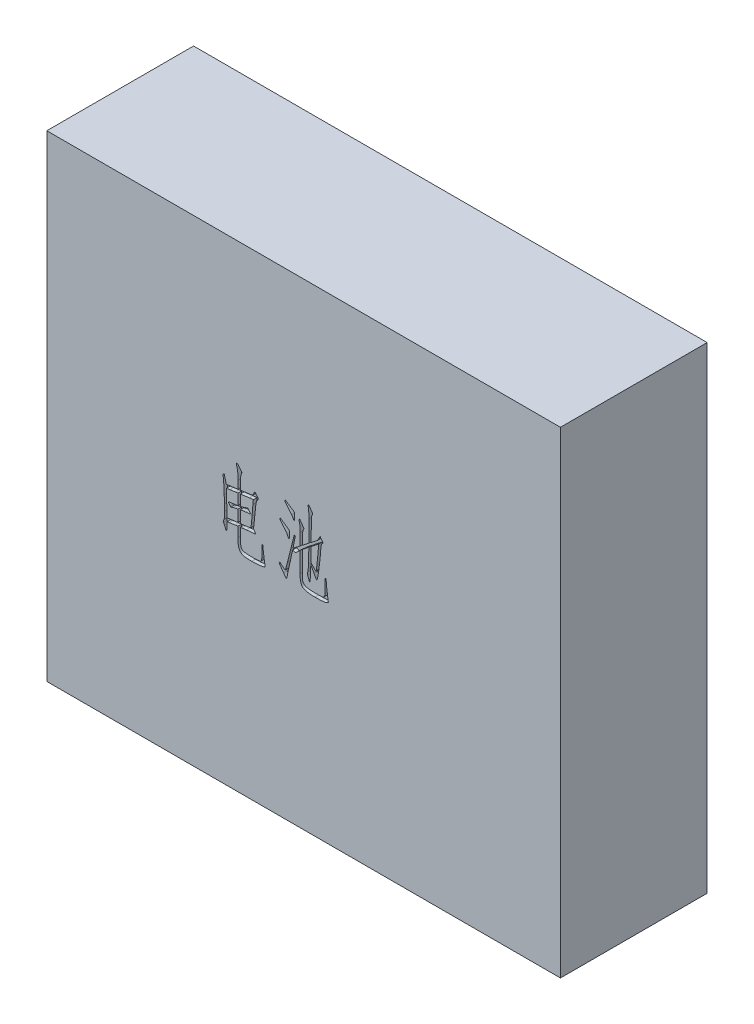
from build123d import *

# Parameters (mm, degrees)
SKETCH1_W           = 70
SKETCH1_H           = 65
BOSS_EXTRUDE1_DEPTH = 20
CUT_EXTRUDE1_DEPTH  = 0.5


with BuildPart() as part:
    # Sketch1 → Boss-Extrude1 (new body)
    with BuildSketch(Plane.XY):
        with Locations((-35, 32.5)):
            Rectangle(SKETCH1_W, SKETCH1_H)
    extrude(amount=BOSS_EXTRUDE1_DEPTH)

    # Sketch2 → Cut-Extrude1 (cut)
    # profile 1 of 4: a face of its own
    with BuildSketch(Plane.XY.offset(20)):
        with BuildLine():
            Line((-45.812964471, 36.577951622), (-45.662953817, 36.013707002))
            Line((-45.662953817, 36.013707002), (-45.536808494, 35.51935371))
            Line((-45.536808494, 35.51935371), (-45.100413864, 35.565379706))
            Line((-45.100413864, 35.565379706), (-44.179893941, 35.679592363))
            Line((-44.179893941, 35.679592363), (-43.937831294, 35.72561836))
            Line((-43.937831294, 35.72561836), (-43.925898629, 36.784216271))
            add(Edge.make_bspline(
                [(-43.925898629, 36.784216271), (-43.925848472, 36.793308603), (-43.925691689, 36.821730497), (-43.928371074, 36.879661448), (-43.929044334, 36.96833947), (-43.933127204, 37.085947103), (-43.937193687, 37.229243594), (-43.947978078, 37.394055669), (-43.963557741, 37.578165031), (-43.983093329, 37.777875129), (-44.010364708, 37.986611595), (-44.052989031, 38.195650038), (-44.109621861, 38.401561451), (-44.15640205, 38.535722825), (-44.179893941, 38.603095453)],
                knots=[0, 0, 0, 0, 0.177294891, 0.554209453, 1.130524385, 1.906506064, 2.848971625, 3.925876191, 5.126764862, 6.452083082, 7.83897123, 9.22979357, 10.608868701, 12, 12, 12, 12], degree=3))
            Line((-44.179893941, 38.603095453), (-44.075909283, 38.763334106))
            Line((-44.075909283, 38.763334106), (-43.38551934, 37.980892172))
            add(Edge.make_bspline(
                [(-43.38551934, 37.980892172), (-43.420264988, 37.902053364), (-43.488395113, 37.747464282), (-43.548848415, 37.540251846), (-43.578172835, 37.355960049), (-43.591770735, 37.182751904), (-43.60237328, 36.972995597), (-43.603245164, 36.820601132), (-43.603716655, 36.738190275)],
                knots=[0, 0, 0, 0, 1.215957117, 2.384278755, 3.034624226, 3.848266097, 4.836399765, 6, 6, 6, 6], degree=3))
            Line((-43.603716655, 36.738190275), (-43.603716655, 35.771644356))
            Line((-43.603716655, 35.771644356), (-43.039472036, 35.841535683))
            Line((-43.039472036, 35.841535683), (-42.154750109, 35.967681006))
            Line((-42.154750109, 35.967681006), (-41.934848128, 36.013707002))
            Line((-41.934848128, 36.013707002), (-41.740516144, 36.416008302))
            add(Edge.make_bspline(
                [(-41.740516144, 36.416008302), (-41.731928078, 36.435064247), (-41.717356021, 36.467397986), (-41.693448368, 36.504929362), (-41.679441503, 36.530548341), (-41.658607454, 36.540135813), (-41.639691378, 36.525794581), (-41.615948836, 36.50712574), (-41.581405092, 36.478434132), (-41.55779387, 36.453777511), (-41.544479494, 36.439873633)],
                knots=[0, 0, 0, 0, 1.663720426, 2.822966936, 3.56700533, 3.954602535, 4.461796658, 5.269494342, 6.4602669, 8, 8, 8, 8], degree=3))
            Line((-41.544479494, 36.439873633), (-41.268323517, 36.129624326))
            add(Edge.make_bspline(
                [(-41.268323517, 36.129624326), (-41.255200499, 36.111510287), (-41.231452655, 36.078730527), (-41.200612861, 36.034289255), (-41.185844914, 35.994837324), (-41.180962255, 35.955454126), (-41.18988266, 35.917798696), (-41.202635799, 35.882495715), (-41.225111729, 35.850918255), (-41.252022896, 35.807221487), (-41.292648636, 35.744473992), (-41.348482267, 35.664851326), (-41.405037234, 35.561917373), (-41.449581952, 35.433292488), (-41.487298387, 35.283335175), (-41.502389125, 35.174648675), (-41.510386163, 35.11705241)],
                knots=[0, 0, 0, 0, 0.847429402, 1.533536147, 2.036930199, 2.426382901, 3.016860564, 3.480069352, 3.837966044, 4.476237987, 5.424607541, 6.665143789, 8.156530738, 9.850434346, 11.801019622, 14, 14, 14, 14], degree=3))
            Line((-41.510386163, 35.11705241), (-41.636531486, 33.92037651))
            Line((-41.636531486, 33.92037651), (-41.78654214, 32.457772632))
            Line((-41.78654214, 32.457772632), (-41.832568136, 32.089564663))
            Line((-41.832568136, 32.089564663), (-41.612666155, 31.779315355))
            add(Edge.make_bspline(
                [(-41.612666155, 31.779315355), (-41.597709173, 31.753286049), (-41.572966997, 31.710227784), (-41.555564052, 31.64939674), (-41.572704739, 31.601362265), (-41.59930459, 31.597267994), (-41.612666155, 31.59521137)],
                knots=[0, 0, 0, 0, 1.606901506, 2.658172752, 3.325977029, 4, 4, 4, 4], degree=3))
            Line((-41.612666155, 31.59521137), (-41.796770139, 31.583278705))
            Line((-41.796770139, 31.583278705), (-42.809342055, 31.491226712))
            Line((-42.809342055, 31.491226712), (-43.38551934, 31.423040051))
            Line((-43.38551934, 31.423040051), (-43.627581987, 31.388946721))
            Line((-43.627581987, 31.388946721), (-43.627581987, 30.146244824))
            add(Edge.make_bspline(
                [(-43.627581987, 30.146244824), (-43.625455316, 30.020075821), (-43.621338914, 29.775861911), (-43.598644778, 29.477145058), (-43.561803409, 29.256634492), (-43.518466195, 29.109417545), (-43.454741682, 28.980941201), (-43.39204268, 28.878371677), (-43.308783505, 28.812143731), (-43.214226104, 28.772149677), (-43.089428354, 28.736815118), (-42.932276864, 28.709423108), (-42.742740398, 28.687794227), (-42.521412057, 28.673764216), (-42.267931823, 28.6629308), (-42.088282823, 28.661983652), (-41.99280679, 28.661480282)],
                knots=[0, 0, 0, 0, 1.931152807, 3.737957541, 4.577172512, 5.350113142, 6.073531508, 6.773090527, 7.162848559, 7.680298175, 8.332476513, 9.14602524, 10.117846342, 11.250994603, 12.539017008, 14, 14, 14, 14], degree=3))
            add(Edge.make_bspline(
                [(-41.99280679, 28.661480282), (-41.903594337, 28.661133851), (-41.735947315, 28.660482842), (-41.501154339, 28.664711566), (-41.29978544, 28.676356186), (-41.132131419, 28.693113532), (-40.996618699, 28.712927385), (-40.895964252, 28.741581905), (-40.822055206, 28.771883437), (-40.756217937, 28.857328089), (-40.726796655, 29.002470979), (-40.711695577, 29.127077752), (-40.704078897, 29.189926904)],
                knots=[0, 0, 0, 0, 1.652015129, 3.104447941, 4.3482727, 5.384821521, 6.227270062, 6.873348196, 7.334536251, 7.663266203, 8.821398446, 10, 10, 10, 10], degree=3))
            Line((-40.704078897, 29.189926904), (-40.704078897, 29.824062851))
            Line((-40.704078897, 29.824062851), (-40.704078897, 30.824702101))
            Line((-40.704078897, 30.824702101), (-40.566000909, 30.846862766))
            Line((-40.566000909, 30.846862766), (-40.543840244, 30.570706789))
            Line((-40.543840244, 30.570706789), (-40.485881582, 30.100218828))
            Line((-40.485881582, 30.100218828), (-40.405762255, 29.478015547))
            Line((-40.405762255, 29.478015547), (-40.323938262, 28.949568924))
            Line((-40.323938262, 28.949568924), (-40.267684267, 28.569428289))
            add(Edge.make_bspline(
                [(-40.267684267, 28.569428289), (-40.261677644, 28.537454545), (-40.252021936, 28.486056413), (-40.248582565, 28.417397749), (-40.27837879, 28.372014815), (-40.307431463, 28.358761234), (-40.323938262, 28.351230974)],
                knots=[0, 0, 0, 0, 1.559608042, 2.507086382, 3.151774227, 4, 4, 4, 4], degree=3))
            Line((-40.323938262, 28.351230974), (-40.415990254, 28.315432977))
            add(Edge.make_bspline(
                [(-40.415990254, 28.315432977), (-40.426712478, 28.311220837), (-40.452204778, 28.30120639), (-40.49889938, 28.290668166), (-40.558255604, 28.276259718), (-40.631918341, 28.263690168), (-40.718618541, 28.24755137), (-40.818903004, 28.233306325), (-40.932319784, 28.215269905), (-41.185704737, 28.182282751), (-41.567309043, 28.143795243), (-41.907463787, 28.143436273), (-42.072926116, 28.143261658)],
                knots=[0, 0, 0, 0, 0.206618915, 0.491240576, 0.857597671, 1.30390666, 1.832361082, 2.441372039, 3.122534554, 3.89462094, 7.030145068, 10, 10, 10, 10], degree=3))
            add(Edge.make_bspline(
                [(-42.072926116, 28.143261658), (-42.164420521, 28.143842078), (-42.337813117, 28.144942042), (-42.583433704, 28.154993204), (-42.800723206, 28.171504943), (-42.990269829, 28.194753914), (-43.152856969, 28.224574619), (-43.287782923, 28.261157691), (-43.396097067, 28.303323646), (-43.497889486, 28.372667533), (-43.591364505, 28.467455716), (-43.686841354, 28.578088586), (-43.76197096, 28.688945914), (-43.832245139, 28.844347638), (-43.885969719, 29.060569894), (-43.931062669, 29.343564055), (-43.955099128, 29.656034013), (-43.958331496, 29.872898525), (-43.959991959, 29.984301505)],
                knots=[0, 0, 0, 0, 1.375107078, 2.605988713, 3.693973982, 4.649466436, 5.475237603, 6.17560074, 6.749778481, 7.211670088, 8.015056038, 8.742243092, 9.407844955, 10.019243034, 11.295622579, 12.740386124, 14.325541172, 16, 16, 16, 16], degree=3))
            Line((-43.959991959, 29.984301505), (-43.959991959, 31.342920725))
            Line((-43.959991959, 31.342920725), (-44.306039264, 31.307122728))
            Line((-44.306039264, 31.307122728), (-45.134507194, 31.180977405))
            Line((-45.134507194, 31.180977405), (-45.432823836, 31.134951409))
            Line((-45.432823836, 31.134951409), (-45.444756502, 30.616732785))
            Line((-45.444756502, 30.616732785), (-45.456689168, 30.318416143))
            add(Edge.make_bspline(
                [(-45.456689168, 30.318416143), (-45.458359636, 30.273533328), (-45.461551521, 30.187772505), (-45.487511175, 30.102103524), (-45.51112075, 30.029386641), (-45.558375641, 30.038317065), (-45.586013212, 30.089408838), (-45.604968918, 30.130530018), (-45.616927821, 30.156472824)],
                knots=[0, 0, 0, 0, 1.721263003, 3.288940973, 3.839377096, 4.198736227, 4.863606649, 6, 6, 6, 6], degree=3))
            Line((-45.616927821, 30.156472824), (-45.790803806, 30.548546124))
            Line((-45.790803806, 30.548546124), (-45.905016464, 30.80083677))
            add(Edge.make_bspline(
                [(-45.905016464, 30.80083677), (-45.916225525, 30.826818695), (-45.934025264, 30.86807741), (-45.962588158, 30.920163424), (-45.950434446, 30.967100334), (-45.933584803, 31.023789903), (-45.899924863, 31.10577543), (-45.873762283, 31.169092752), (-45.858990467, 31.204842736)],
                knots=[0, 0, 0, 0, 1.195724136, 1.898783123, 2.330290027, 3.145663464, 4.388395428, 6, 6, 6, 6], degree=3))
            add(Edge.make_bspline(
                [(-45.858990467, 31.204842736), (-45.849809434, 31.226217303), (-45.830217739, 31.271829156), (-45.812969093, 31.350842435), (-45.798550733, 31.441839518), (-45.794928356, 31.578213425), (-45.791037076, 31.745202497), (-45.786619115, 31.927653626), (-45.780327837, 32.074186752), (-45.779294197, 32.158883823), (-45.778871141, 32.193549321)],
                knots=[0, 0, 0, 0, 0.558699634, 1.192226558, 1.938775613, 2.774002823, 4.470288396, 5.961506424, 7.165668957, 8, 8, 8, 8], degree=3))
            Line((-45.778871141, 32.193549321), (-45.790803806, 33.056110582))
            Line((-45.790803806, 33.056110582), (-45.824897137, 34.138573825))
            add(Edge.make_bspline(
                [(-45.824897137, 34.138573825), (-45.824797251, 34.152212755), (-45.824559958, 34.184613823), (-45.827034133, 34.2397075), (-45.828061889, 34.308497074), (-45.831764637, 34.390323987), (-45.837314584, 34.486300534), (-45.842238946, 34.595980451), (-45.846952964, 34.719327295), (-45.856167901, 34.894310057), (-45.866887814, 35.102277761), (-45.877722314, 35.324559799), (-45.890900336, 35.502261385), (-45.899135518, 35.652460744), (-45.913678834, 35.80572857), (-45.929393585, 35.994614848), (-45.956882817, 36.234104167), (-45.975113007, 36.410873963), (-45.98513579, 36.508060294)],
                knots=[0, 0, 0, 0, 0.275532466, 0.654563513, 1.113927774, 1.665470852, 2.30930182, 3.056329963, 3.883644582, 4.803233469, 6.596547928, 8.091177521, 9.299307877, 10.196626331, 11.130014446, 12.409513054, 14.025984863, 16, 16, 16, 16], degree=3))
            Line((-45.98513579, 36.508060294), (-45.812964471, 36.577951622))
        make_face()
        with BuildLine():
            Line((-45.432823836, 31.607144036), (-43.959991959, 31.779315355))
            Line((-43.959991959, 31.779315355), (-43.94976396, 33.378292555))
            Line((-43.94976396, 33.378292555), (-44.260013267, 33.310105894))
            Line((-44.260013267, 33.310105894), (-44.616288571, 33.218053902))
            Line((-44.616288571, 33.218053902), (-44.938470544, 33.102136578))
            Line((-44.938470544, 33.102136578), (-45.018589871, 33.218053902))
            Line((-45.018589871, 33.218053902), (-45.214626521, 33.470344547))
            add(Edge.make_bspline(
                [(-45.214626521, 33.470344547), (-45.22660598, 33.483568984), (-45.247192553, 33.506295039), (-45.261151514, 33.549702385), (-45.239906849, 33.586199824), (-45.215591355, 33.594037338), (-45.202693855, 33.598194537)],
                knots=[0, 0, 0, 0, 1.284117706, 2.206742812, 3.048814964, 4, 4, 4, 4], degree=3))
            Line((-45.202693855, 33.598194537), (-44.800392556, 33.654448532))
            Line((-44.800392556, 33.654448532), (-44.328199928, 33.712407194))
            Line((-44.328199928, 33.712407194), (-43.94976396, 33.782298521))
            Line((-43.94976396, 33.782298521), (-43.937831294, 35.277291064))
            Line((-43.937831294, 35.277291064), (-44.282173932, 35.219332402))
            Line((-44.282173932, 35.219332402), (-45.054387868, 35.11705241))
            Line((-45.054387868, 35.11705241), (-45.524875829, 35.035228417))
            Line((-45.524875829, 35.035228417), (-45.502715164, 34.138573825))
            Line((-45.502715164, 34.138573825), (-45.432823836, 31.607144036))
        make_face(mode=Mode.SUBTRACT)
        with BuildLine():
            Line((-43.627581987, 31.825341351), (-42.799114056, 31.917393344))
            Line((-42.799114056, 31.917393344), (-42.407040755, 31.987284671))
            Line((-42.407040755, 31.987284671), (-42.176910774, 32.033310667))
            Line((-42.176910774, 32.033310667), (-42.118952112, 32.585622621))
            Line((-42.118952112, 32.585622621), (-42.02690012, 33.516370544))
            Line((-42.02690012, 33.516370544), (-41.912687463, 34.92101576))
            Line((-41.912687463, 34.92101576), (-41.854728801, 35.531286376))
            Line((-41.854728801, 35.531286376), (-42.395108089, 35.473327714))
            Line((-42.395108089, 35.473327714), (-43.615649321, 35.311384394))
            Line((-43.615649321, 35.311384394), (-43.627581987, 33.850485182))
            add(Edge.make_bspline(
                [(-43.627581987, 33.850485182), (-43.518158759, 33.876588548), (-43.314629368, 33.925141329), (-43.03688824, 34.009381589), (-42.805865185, 34.08904511), (-42.674156189, 34.154987357), (-42.615010071, 34.184599821)],
                knots=[0, 0, 0, 0, 1.262396956, 2.348083582, 3.25817942, 4, 4, 4, 4], degree=3))
            Line((-42.615010071, 34.184599821), (-42.303056097, 33.804459186))
            add(Edge.make_bspline(
                [(-42.303056097, 33.804459186), (-42.287987807, 33.780864519), (-42.262053617, 33.740255495), (-42.244999942, 33.678242919), (-42.26725058, 33.626405214), (-42.298551095, 33.6224384), (-42.314988763, 33.620355202)],
                knots=[0, 0, 0, 0, 1.442479735, 2.482666664, 3.203162602, 4, 4, 4, 4], degree=3))
            Line((-42.314988763, 33.620355202), (-42.476932083, 33.608422536))
            Line((-42.476932083, 33.608422536), (-42.855368051, 33.56239654))
            Line((-42.855368051, 33.56239654), (-43.22357602, 33.516370544))
            Line((-43.22357602, 33.516370544), (-43.627581987, 33.436251217))
            Line((-43.627581987, 33.436251217), (-43.627581987, 31.825341351))
        make_face(mode=Mode.SUBTRACT)
    # profile 2 of 4: a face of its own
    with BuildSketch(Plane.XY.offset(20)):
        with BuildLine():
            Line((-36.266831933, 34.16073449), (-36.128753945, 34.092547829))
            Line((-36.128753945, 34.092547829), (-36.198645272, 33.75843319))
            Line((-36.198645272, 33.75843319), (-36.450935918, 32.503798628))
            Line((-36.450935918, 32.503798628), (-35.474162, 33.240214567))
            Line((-35.474162, 33.240214567), (-35.474162, 34.874989764))
            add(Edge.make_bspline(
                [(-35.474162, 34.874989764), (-35.476014604, 34.96137645), (-35.479489325, 35.123402178), (-35.490539761, 35.349501037), (-35.500546316, 35.543024737), (-35.524060765, 35.755403005), (-35.560200686, 35.996883008), (-35.617784828, 36.177939791), (-35.646333318, 36.267702314)],
                knots=[0, 0, 0, 0, 1.103429514, 2.069577835, 2.891178562, 3.577175633, 4.798836336, 6, 6, 6, 6], degree=3))
            Line((-35.646333318, 36.267702314), (-35.54234866, 36.405780303))
            Line((-35.54234866, 36.405780303), (-34.955943376, 35.577312372))
            add(Edge.make_bspline(
                [(-34.955943376, 35.577312372), (-34.974187002, 35.535505071), (-35.008613632, 35.456612614), (-35.047899028, 35.341111526), (-35.084247663, 35.239951635), (-35.111919704, 35.121866565), (-35.134793499, 34.98830644), (-35.148705642, 34.833197358), (-35.151718217, 34.673813064), (-35.156499279, 34.53809038), (-35.158834538, 34.433999815), (-35.159376391, 34.376731057), (-35.157831897, 34.341522739), (-35.153209175, 34.326636069), (-35.151980026, 34.32267781)],
                knots=[0, 0, 0, 0, 1.277874718, 2.411413148, 3.418754168, 4.287932458, 5.8066473, 7.214043668, 8.648311221, 10.273614673, 11.022374716, 11.563908357, 11.884046341, 12, 12, 12, 12], degree=3))
            Line((-35.151980026, 34.32267781), (-35.151980026, 33.506142545))
            Line((-35.151980026, 33.506142545), (-34.287714098, 34.172667156))
            Line((-34.287714098, 34.172667156), (-34.265553434, 37.060372248))
            add(Edge.make_bspline(
                [(-34.265553434, 37.060372248), (-34.265567288, 37.080828343), (-34.265606541, 37.138787278), (-34.265162028, 37.226295863), (-34.266854845, 37.335473149), (-34.275011468, 37.46155569), (-34.28448686, 37.625286771), (-34.299716924, 37.815015709), (-34.315236821, 38.006585831), (-34.331193271, 38.175590104), (-34.350006539, 38.309063556), (-34.363687497, 38.386063025), (-34.369538092, 38.418991468)],
                knots=[0, 0, 0, 0, 0.449890352, 1.274689332, 1.924651104, 2.850775754, 4.052824256, 5.531747845, 7.036580408, 8.280074453, 9.264482312, 10, 10, 10, 10], degree=3))
            Line((-34.369538092, 38.418991468), (-34.415564088, 38.625256118))
            Line((-34.415564088, 38.625256118), (-34.287714098, 38.68321478))
            Line((-34.287714098, 38.68321478), (-33.74733481, 37.900772845))
            add(Edge.make_bspline(
                [(-33.74733481, 37.900772845), (-33.766404625, 37.866289513), (-33.802202035, 37.801558211), (-33.847870249, 37.707751639), (-33.878165259, 37.622902765), (-33.899502497, 37.543742215), (-33.908881892, 37.458884191), (-33.915467155, 37.359370748), (-33.918190644, 37.239371454), (-33.919045193, 37.152991043), (-33.919506129, 37.106398244)],
                knots=[0, 0, 0, 0, 1.143336114, 2.146243721, 3.022303475, 3.754005903, 4.518761241, 5.493636838, 6.648090788, 8, 8, 8, 8], degree=3))
            Line((-33.919506129, 37.106398244), (-33.955304126, 36.335888975))
            Line((-33.955304126, 36.335888975), (-33.977464791, 34.414729802))
            Line((-33.977464791, 34.414729802), (-33.068877533, 35.127280409))
            Line((-33.068877533, 35.127280409), (-32.872840883, 35.51935371))
            add(Edge.make_bspline(
                [(-32.872840883, 35.51935371), (-32.856433799, 35.552914195), (-32.82830764, 35.6104459), (-32.792135435, 35.682424601), (-32.770561775, 35.725618797), (-32.760901283, 35.744937997), (-32.758628226, 35.749483691)],
                knots=[0, 0, 0, 0, 1.744829883, 2.991108106, 3.762613672, 4, 4, 4, 4], degree=3))
            Line((-32.758628226, 35.749483691), (-32.676804233, 35.633566367))
            Line((-32.676804233, 35.633566367), (-32.458606917, 35.32331706))
            add(Edge.make_bspline(
                [(-32.458606917, 35.32331706), (-32.443653988, 35.302994829), (-32.417026915, 35.266806498), (-32.385056675, 35.218752815), (-32.365333603, 35.184146801), (-32.359121369, 35.156885985), (-32.368895301, 35.133542169), (-32.390568064, 35.110843652), (-32.415360258, 35.075245581), (-32.471571134, 35.026430074), (-32.533300526, 34.940260201), (-32.58332619, 34.817342596), (-32.613550103, 34.687073492), (-32.637155762, 34.574525941), (-32.647320913, 34.467048566), (-32.65797822, 34.35179159), (-32.667177907, 34.199368585), (-32.677326232, 34.048262427), (-32.685007695, 33.904931773), (-32.696276797, 33.776627085), (-32.707394313, 33.631611698), (-32.723623656, 33.469796301), (-32.740012444, 33.290688105), (-32.760661301, 33.094660481), (-32.784934581, 32.882253834), (-32.81776993, 32.583157902), (-32.86262768, 32.216139844), (-32.914711884, 31.797743919), (-32.967462662, 31.416422779), (-33.01173421, 31.123828042), (-33.047253659, 30.914378011), (-33.070368655, 30.781720304), (-33.093760988, 30.669020712), (-33.117931343, 30.576517991), (-33.139457992, 30.503551831), (-33.158917083, 30.449578549), (-33.178033124, 30.415054976), (-33.204460577, 30.392853951), (-33.241329818, 30.400660804), (-33.277931363, 30.424922015), (-33.313838902, 30.468260951), (-33.33381771, 30.504395439), (-33.34503351, 30.524680793)],
                knots=[0, 0, 0, 0, 0.572960633, 1.020286037, 1.308793021, 1.47849792, 1.629516928, 1.859238066, 2.189701376, 2.609377403, 3.540946753, 4.564231855, 5.603177511, 6.574893703, 7.171901031, 8.052674627, 9.203596934, 10.638611067, 11.491733585, 12.46250707, 13.562925808, 14.794144362, 16.155029084, 17.646864078, 19.269751124, 21.009474552, 24.479075422, 27.665373512, 30.5830622, 33.219864516, 34.384375344, 35.406846701, 36.277354076, 36.997119736, 37.576724451, 38.005620917, 38.295566847, 38.471058794, 38.743235739, 39.061902118, 39.473366081, 40, 40, 40, 40], degree=3))
            Line((-33.34503351, 30.524680793), (-33.587096157, 30.984940755))
            Line((-33.587096157, 30.984940755), (-33.885412799, 31.515092044))
            Line((-33.885412799, 31.515092044), (-34.023490787, 31.745222025))
            Line((-34.023490787, 31.745222025), (-34.057584118, 30.674691447))
            Line((-34.057584118, 30.674691447), (-34.103610114, 29.972368839))
            add(Edge.make_bspline(
                [(-34.103610114, 29.972368839), (-34.106429464, 29.934450286), (-34.111445377, 29.866989299), (-34.118331654, 29.776130099), (-34.136427813, 29.715454841), (-34.146112218, 29.667009521), (-34.189496201, 29.656430258), (-34.216489732, 29.713246126), (-34.251617239, 29.784219805), (-34.274228258, 29.851889453), (-34.287714098, 29.892249512)],
                knots=[0, 0, 0, 0, 1.548277697, 2.75454446, 3.632054474, 4.21957732, 4.527029857, 5.164410394, 6.308775526, 8, 8, 8, 8], degree=3))
            Line((-34.287714098, 29.892249512), (-34.449657418, 30.306483478))
            add(Edge.make_bspline(
                [(-34.449657418, 30.306483478), (-34.458630314, 30.329060699), (-34.474645019, 30.369356226), (-34.490058561, 30.424263975), (-34.504244789, 30.463715075), (-34.508970445, 30.495701665), (-34.504239928, 30.527686838), (-34.490277835, 30.566634975), (-34.47499331, 30.619937311), (-34.446190036, 30.684986815), (-34.419284066, 30.768308992), (-34.397550669, 30.872269511), (-34.381675766, 30.996582431), (-34.368686227, 31.135932694), (-34.3598749, 31.279274473), (-34.349848348, 31.414962542), (-34.347330571, 31.538381859), (-34.346206164, 31.616236764), (-34.34567276, 31.653170032)],
                knots=[0, 0, 0, 0, 0.847620795, 1.512822455, 1.989839709, 2.309771091, 2.629702473, 3.106719727, 3.753010358, 4.563594937, 5.586336595, 6.804437419, 8.266379239, 9.96034311, 11.690636616, 13.281037962, 14.71016275, 16, 16, 16, 16], degree=3))
            Line((-34.34567276, 31.653170032), (-34.287714098, 33.700474528))
            Line((-34.287714098, 33.700474528), (-35.151980026, 33.010084586))
            Line((-35.151980026, 33.010084586), (-35.174140691, 30.122379493))
            add(Edge.make_bspline(
                [(-35.174140691, 30.122379493), (-35.174140472, 30.115560828), (-35.17413987, 30.0968095), (-35.174148598, 30.059306784), (-35.174087003, 30.004757827), (-35.174429939, 29.931449836), (-35.172579481, 29.838797384), (-35.167835228, 29.723921765), (-35.155337701, 29.586034783), (-35.148882248, 29.430800344), (-35.119381123, 29.269799603), (-35.044165651, 29.122854344), (-34.931090073, 28.997709282), (-34.808317108, 28.912174159), (-34.688969348, 28.858162305), (-34.581804486, 28.820401233), (-34.459276254, 28.788287813), (-34.32118352, 28.763912688), (-34.168307845, 28.742717205), (-33.999787323, 28.730307966), (-33.815614193, 28.721514998), (-33.687683782, 28.720148965), (-33.621189487, 28.719438943)],
                knots=[0, 0, 0, 0, 0.160723151, 0.441988665, 0.883977329, 1.446508357, 2.169886539, 3.068156583, 4.156010134, 5.431851206, 6.732134165, 7.978026584, 9.268268598, 10.672745357, 11.469748722, 12.350880404, 13.348231265, 14.451557942, 15.654374443, 16.984662635, 18.432720347, 20, 20, 20, 20], degree=3))
            add(Edge.make_bspline(
                [(-33.621189487, 28.719438943), (-33.550731062, 28.718760795), (-33.416066642, 28.717464678), (-33.224562404, 28.717334614), (-33.052963938, 28.719256917), (-32.901155872, 28.721523233), (-32.769422857, 28.729529557), (-32.65725881, 28.734901764), (-32.565727993, 28.745197424), (-32.472846567, 28.759877815), (-32.380592014, 28.785778443), (-32.288133409, 28.821066771), (-32.219111079, 28.868162134), (-32.167579013, 28.924731454), (-32.138225494, 28.999698933), (-32.111878457, 29.08944655), (-32.099049201, 29.20219639), (-32.093446093, 29.283687485), (-32.090398948, 29.328004893)],
                knots=[0, 0, 0, 0, 1.766276756, 3.375815332, 4.800256971, 6.068266689, 7.180735551, 8.10832774, 8.882221105, 9.488708597, 10.463127887, 11.28049811, 11.956136324, 12.541689444, 13.166467087, 13.951035347, 14.885708911, 16, 16, 16, 16], degree=3))
            Line((-32.090398948, 29.328004893), (-32.090398948, 30.904821428))
            Line((-32.090398948, 30.904821428), (-32.090398948, 31.146884074))
            Line((-32.090398948, 31.146884074), (-31.95232096, 31.169044739))
            Line((-31.95232096, 31.169044739), (-31.906294963, 30.754810774))
            Line((-31.906294963, 30.754810774), (-31.848336302, 30.122379493))
            Line((-31.848336302, 30.122379493), (-31.722190979, 29.121740243))
            add(Edge.make_bspline(
                [(-31.722190979, 29.121740243), (-31.716410034, 29.071180568), (-31.706081299, 28.980846285), (-31.693670807, 28.861215467), (-31.680473943, 28.77363014), (-31.664727261, 28.700393767), (-31.647391817, 28.632678288), (-31.632702925, 28.570288193), (-31.643437061, 28.51575527), (-31.682937455, 28.478454086), (-31.738537519, 28.435842095), (-31.786920213, 28.411182678), (-31.814242971, 28.39725697)],
                knots=[0, 0, 0, 0, 1.862405269, 3.327534118, 4.401050164, 5.102555638, 6.065884989, 6.968735006, 7.417638403, 8.022127244, 8.88305229, 10, 10, 10, 10], degree=3))
            add(Edge.make_bspline(
                [(-31.814242971, 28.39725697), (-31.847473307, 28.382794897), (-31.9223428, 28.350211171), (-32.054525999, 28.316858225), (-32.215257185, 28.288611423), (-32.405445074, 28.265795085), (-32.624744914, 28.244856909), (-32.873836847, 28.231893647), (-33.151809015, 28.226061559), (-33.34673584, 28.224303485), (-33.449018168, 28.223380985)],
                knots=[0, 0, 0, 0, 0.525453063, 1.183870223, 1.971909494, 2.89486667, 3.96365597, 5.169900272, 6.514985356, 8, 8, 8, 8], degree=3))
            add(Edge.make_bspline(
                [(-33.449018168, 28.223380985), (-33.581475292, 28.223124504), (-33.833128402, 28.222637221), (-34.189161325, 28.252070607), (-34.503177112, 28.29961452), (-34.736660285, 28.358982933), (-34.899755786, 28.421003055), (-35.004939115, 28.476836508), (-35.099995186, 28.53868782), (-35.179742553, 28.61340677), (-35.249742785, 28.693428265), (-35.30437983, 28.784573832), (-35.349384388, 28.882593329), (-35.386342098, 29.019989162), (-35.41721705, 29.180048089), (-35.450264942, 29.347594644), (-35.472989564, 29.479358065), (-35.48959416, 29.602024959), (-35.492070822, 29.718379301), (-35.497044353, 29.829143167), (-35.496248969, 29.907024944), (-35.496303671, 29.947935712), (-35.496322664, 29.96214084)],
                knots=[0, 0, 0, 0, 2.462684528, 4.67881384, 6.636999054, 8.364825419, 9.147899839, 9.875905864, 10.576468373, 11.249712985, 11.901975396, 12.547265221, 13.219015024, 13.901323428, 15.186439089, 16.251823802, 17.077121389, 17.673568011, 18.551778676, 19.239061844, 19.735785362, 20, 20, 20, 20], degree=3))
            Line((-35.496322664, 29.96214084), (-35.474162, 32.72370061))
            add(Edge.make_bspline(
                [(-35.474162, 32.72370061), (-35.582177534, 32.63179892), (-35.795245885, 32.450516277), (-35.987793051, 32.247580367), (-36.082727949, 32.147523324)],
                knots=[0, 0, 0, 0, 1.013905004, 2, 2, 2, 2], degree=3))
            Line((-36.082727949, 32.147523324), (-36.496961914, 32.273668647))
            Line((-36.496961914, 32.273668647), (-36.808915888, 30.824702101))
            Line((-36.808915888, 30.824702101), (-37.165191192, 29.20185957))
            Line((-37.165191192, 29.20185957), (-37.233377853, 28.845584266))
            add(Edge.make_bspline(
                [(-37.233377853, 28.845584266), (-37.246794197, 28.787677115), (-37.269791443, 28.688417212), (-37.307409568, 28.556899267), (-37.324017813, 28.492978289), (-37.349845784, 28.441009346), (-37.372346316, 28.462343518), (-37.391314575, 28.486379095), (-37.42544239, 28.525943153), (-37.465087201, 28.581707099), (-37.519292286, 28.650562432), (-37.57882964, 28.738031645), (-37.651423725, 28.83848414), (-37.70225484, 28.910864763), (-37.729435812, 28.949568924)],
                knots=[0, 0, 0, 0, 2.07497586, 3.55676105, 4.466827747, 4.800211812, 4.968619417, 5.357211501, 5.941249148, 6.724328603, 7.73059332, 8.952705414, 10.370517209, 12, 12, 12, 12], degree=3))
            Line((-37.729435812, 28.949568924), (-38.257882434, 29.696212862))
            Line((-38.257882434, 29.696212862), (-38.349934427, 29.846223516))
            Line((-38.349934427, 29.846223516), (-38.281747766, 29.99623417))
            Line((-38.281747766, 29.99623417), (-38.165830442, 29.904182178))
            Line((-38.165830442, 29.904182178), (-37.775461808, 29.570067539))
            add(Edge.make_bspline(
                [(-37.775461808, 29.570067539), (-37.744311019, 29.54386298), (-37.689619759, 29.497855787), (-37.617952476, 29.432605449), (-37.569370165, 29.40477681), (-37.529600568, 29.369246809), (-37.507385765, 29.40848859), (-37.488548319, 29.456253362), (-37.458827166, 29.545320775), (-37.422995419, 29.665718967), (-37.375571655, 29.822434979), (-37.323927196, 30.0141315), (-37.264482481, 30.241110604), (-37.222004367, 30.403651067), (-37.199284522, 30.490587462)],
                knots=[0, 0, 0, 0, 1.003500883, 1.761840696, 2.269784058, 2.548928131, 2.726560793, 3.180073805, 3.912603369, 4.956880628, 6.27350926, 7.898819114, 9.806442298, 12, 12, 12, 12], degree=3))
            Line((-37.199284522, 30.490587462), (-36.370816591, 33.75843319))
            Line((-36.370816591, 33.75843319), (-36.266831933, 34.16073449))
        make_face()
        with BuildLine():
            Line((-34.023490787, 32.043538666), (-33.885412799, 31.895232679))
            add(Edge.make_bspline(
                [(-33.885412799, 31.895232679), (-33.842815042, 31.851459554), (-33.763223454, 31.769671854), (-33.651965646, 31.655920249), (-33.559776698, 31.557739713), (-33.479393502, 31.481373088), (-33.418611321, 31.41969568), (-33.371148497, 31.378891692), (-33.342193485, 31.352705851), (-33.325789623, 31.345071534), (-33.321168179, 31.342920725)],
                knots=[0, 0, 0, 0, 1.853692376, 3.463523279, 4.829501388, 5.939248689, 6.829515306, 7.452499084, 7.845753089, 8, 8, 8, 8], degree=3))
            add(Edge.make_bspline(
                [(-33.321168179, 31.342920725), (-33.318686316, 31.345660209), (-33.309435275, 31.35587152), (-33.30826821, 31.387061019), (-33.2944001, 31.431888441), (-33.289768994, 31.469402762), (-33.287074848, 31.491226712)],
                knots=[0, 0, 0, 0, 0.284593498, 1.060810166, 2.290126812, 4, 4, 4, 4], degree=3))
            Line((-33.287074848, 31.491226712), (-33.195022856, 32.067403998))
            add(Edge.make_bspline(
                [(-33.195022856, 32.067403998), (-33.192184436, 32.088428238), (-33.185819334, 32.135574698), (-33.175180731, 32.213875141), (-33.165668728, 32.307784934), (-33.153459222, 32.417418904), (-33.139631107, 32.542919305), (-33.126095128, 32.684426726), (-33.112846368, 32.84190968), (-33.091647556, 33.079411416), (-33.063012492, 33.404517597), (-33.023656918, 33.82328773), (-32.979269359, 34.278997937), (-32.947378317, 34.594866205), (-32.930799545, 34.75907244)],
                knots=[0, 0, 0, 0, 0.282374592, 0.63321965, 1.051652618, 1.538571367, 2.101494521, 2.732132824, 3.430554687, 4.204978052, 5.905829834, 7.77444246, 9.803315611, 12, 12, 12, 12], degree=3))
            Line((-32.930799545, 34.75907244), (-33.977464791, 33.942537175))
            Line((-33.977464791, 33.942537175), (-34.023490787, 32.043538666))
        make_face(mode=Mode.SUBTRACT)
    # profile 3 of 4: a face of its own
    with BuildSketch(Plane.XY.offset(20)):
        with BuildLine():
            Line((-38.257882434, 35.035228417), (-38.211856438, 35.209104403))
            Line((-38.211856438, 35.209104403), (-38.039685119, 35.105119745))
            Line((-38.039685119, 35.105119745), (-37.487373165, 34.736911775))
            Line((-37.487373165, 34.736911775), (-37.165191192, 34.51871446))
            add(Edge.make_bspline(
                [(-37.165191192, 34.51871446), (-37.139579713, 34.49890189), (-37.092915468, 34.462803289), (-37.030603448, 34.41316022), (-36.98758587, 34.368752196), (-36.957657044, 34.329818377), (-36.94162008, 34.287214586), (-36.929655002, 34.236953258), (-36.923647087, 34.174506978), (-36.923309522, 34.128920459), (-36.923128545, 34.104480495)],
                knots=[0, 0, 0, 0, 1.522383335, 2.773790129, 3.737000143, 4.42615918, 5.060914814, 5.857582761, 6.851401605, 8, 8, 8, 8], degree=3))
            Line((-36.923128545, 34.104480495), (-36.935061211, 33.56239654))
            add(Edge.make_bspline(
                [(-36.935061211, 33.56239654), (-36.938292473, 33.525394624), (-36.943555616, 33.465125177), (-36.957388802, 33.391369162), (-37.004941101, 33.34828598), (-37.033759301, 33.367791541), (-37.049273868, 33.378292555)],
                knots=[0, 0, 0, 0, 1.627882292, 2.651526639, 3.274035803, 4, 4, 4, 4], degree=3))
            add(Edge.make_bspline(
                [(-37.049273868, 33.378292555), (-37.058877624, 33.386987166), (-37.084643193, 33.410313625), (-37.113107387, 33.472055533), (-37.158165272, 33.556619397), (-37.192489688, 33.654765356), (-37.239711023, 33.75530112), (-37.305757784, 33.854388137), (-37.390455967, 33.979991425), (-37.501888503, 34.127048885), (-37.637115909, 34.297660427), (-37.795846598, 34.491872814), (-37.978309302, 34.710035831), (-38.108849306, 34.862623413), (-38.177763108, 34.943176425)],
                knots=[0, 0, 0, 0, 0.238677714, 0.640339848, 1.239453301, 2.024919797, 2.562772758, 3.297367404, 4.230686253, 5.376218849, 6.72047884, 8.272350081, 10.032124092, 12, 12, 12, 12], degree=3))
            Line((-38.177763108, 34.943176425), (-38.257882434, 35.035228417))
        make_face()
    # profile 4 of 4: a face of its own
    with BuildSketch(Plane.XY.offset(20)):
        with BuildLine():
            Line((-37.567492492, 37.464378215), (-37.50953383, 37.658710198))
            Line((-37.50953383, 37.658710198), (-37.349295177, 37.556430207))
            Line((-37.349295177, 37.556430207), (-36.808915888, 37.210382902))
            Line((-36.808915888, 37.210382902), (-36.370816591, 36.92229426))
            add(Edge.make_bspline(
                [(-36.370816591, 36.92229426), (-36.343722772, 36.901078419), (-36.294781742, 36.862755099), (-36.245199148, 36.785325286), (-36.222672511, 36.693451547), (-36.221484175, 36.627516457), (-36.220805937, 36.589884288)],
                knots=[0, 0, 0, 0, 1.072235441, 1.936836859, 2.82245848, 4, 4, 4, 4], degree=3))
            Line((-36.220805937, 36.589884288), (-36.220805937, 36.013707002))
            add(Edge.make_bspline(
                [(-36.220805937, 36.013707002), (-36.222316293, 35.982227746), (-36.224762438, 35.931244474), (-36.235248513, 35.864618197), (-36.283464618, 35.83370371), (-36.309724877, 35.85276229), (-36.324790595, 35.863696348)],
                knots=[0, 0, 0, 0, 1.57672254, 2.553633218, 3.170207904, 4, 4, 4, 4], degree=3))
            Line((-36.324790595, 35.863696348), (-36.428775253, 36.037572334))
            Line((-36.428775253, 36.037572334), (-36.646972568, 36.381914972))
            add(Edge.make_bspline(
                [(-36.646972568, 36.381914972), (-36.661567617, 36.403070024), (-36.699855281, 36.458566757), (-36.777036837, 36.55563872), (-36.885313414, 36.687771265), (-37.016425056, 36.843221951), (-37.14959376, 37.00359921), (-37.271684182, 37.143623484), (-37.369708343, 37.255815166), (-37.428214742, 37.320674219), (-37.453279835, 37.348460891)],
                knots=[0, 0, 0, 0, 0.489752707, 1.284784106, 2.362250947, 3.746125377, 5.160514092, 6.335211891, 7.286777722, 8, 8, 8, 8], degree=3))
            Line((-37.453279835, 37.348460891), (-37.567492492, 37.464378215))
        make_face()
    extrude(amount=-CUT_EXTRUDE1_DEPTH, mode=Mode.SUBTRACT)


solid = part.part
